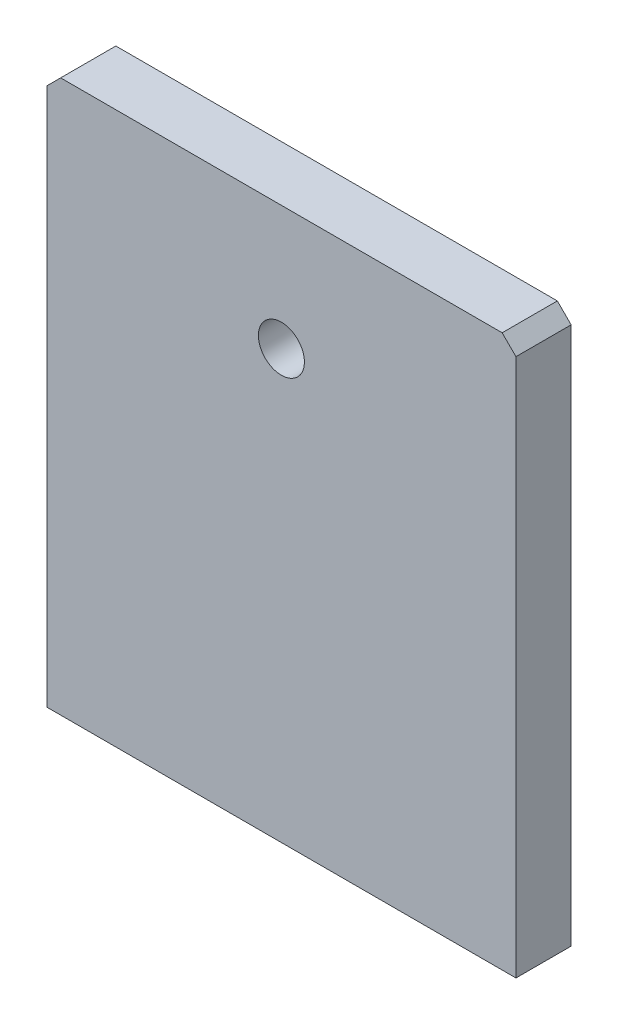
SolidWorks part; units mm, degrees
material "Q235"
ref_plane "Front Plane" through (0, 0, 0) normal (0, 0, 1) x (1, 0, 0)
ref_plane "Top Plane" through (0, 0, 0) normal (0, 1, 0) x (1, 0, 0)
ref_plane "Right Plane" through (0, 0, 0) normal (1, 0, 0) x (0, 0, -1)
sketch "Sketch1" plane through (0, 0, 0) normal (0, 0, 1) x (1, 0, 0)
  line L0 (0, 195) -> (5, 200)
  line L1 (0, 0) -> (170, 0)
  line L2 (0, 0) -> (0, 195)
  line L3 (5, 200) -> (165, 200)
  line L4 (170, 0) -> (170, 195)
  line L5 (165, 200) -> (170, 195)
  point P1 (170, 200)
  point P2 (0, 200)
  dimension "D1" = 200
  dimension "D2" = 170
extrude "Boss-Extrude1" add sketch "Sketch1" along normal blind 20
hole_wizard "3/4-10 Tapped Hole1" positions "3DSketch1" profile "Sketch2" tap size "3/4-10" standard "Progressive" end condition through all
sketch3d "3DSketch1"
  line L0 (0, 0, 20) -> (170, 0, 20) construction
  line L1 (0, 195, 20) -> (0, 0, 20) construction
  point P0 (85, 155, 20)
  dimension "D1" = 155
  dimension "D2" = 85
sketch "Sketch2" plane through (85, 155, 20) normal (1, 0, 0) x (0, -1, 0)
  line L0 (0, 0) -> (0, 20)
  line L1 (0, 20) -> (8.3337, 20)
  line L2 (8.3337, 20) -> (8.3337, 0)
  line L5 (8.3337, 0) -> (0, 0)
  line L11 (0, -6.35) -> (0, 107.95) construction
  dimension "通孔螺纹孔钻头直径" = 16.6675
  dimension "通孔螺纹孔钻头深度" = 20
cosmetic thread "Cosmetic thread 1"
